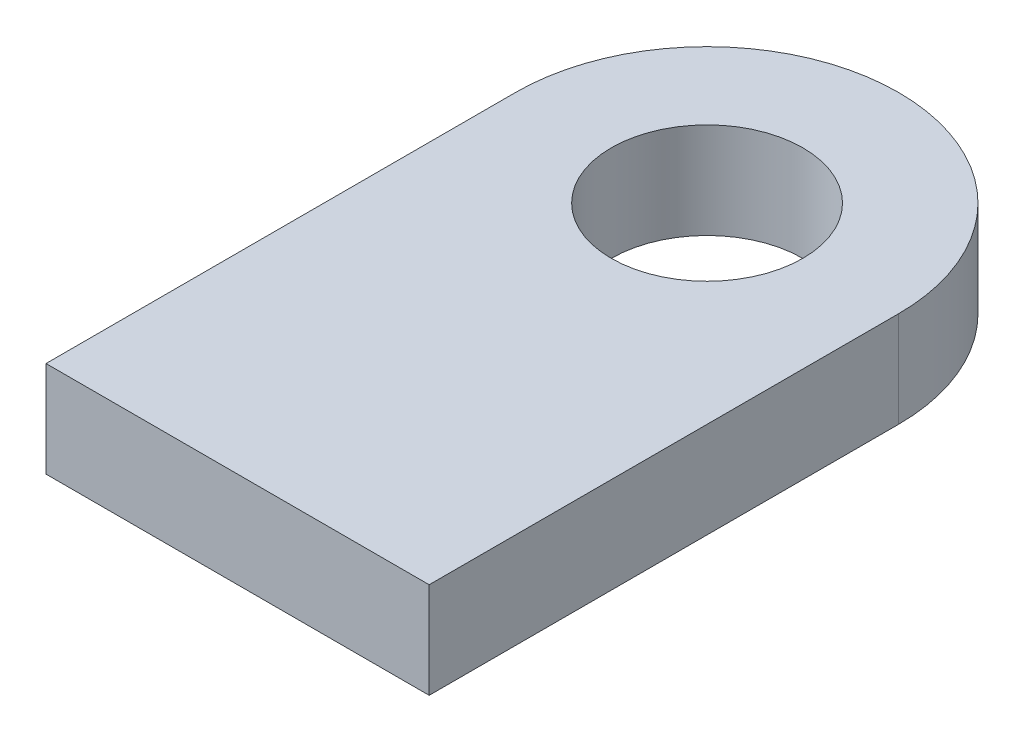
from build123d import *

# Parameters (mm, degrees)
SKETCH_1_R      = 10
EXTRUDE_1_DEPTH = 5


with BuildPart() as part:
    # 草图1 → 凸台-拉伸1 (new, symmetric)
    with BuildSketch(Plane(origin=(0, 0, 0), x_dir=(1, 0, 0), z_dir=(0, 1, 0))):
        with BuildLine():
            Line((-20, -24.505), (20, -24.505))
            Line((20, -24.505), (20, 24.505))
            ThreePointArc((20, 24.505), (0, 44.505), (-20, 24.505))
            Line((-20, 24.505), (-20, -24.505))
        make_face()
        with Locations(Location((0, 24.505, 0), (0, 0, 270))):
            Circle(SKETCH_1_R, mode=Mode.SUBTRACT)
    extrude(amount=EXTRUDE_1_DEPTH, both=True)


solid = part.part
